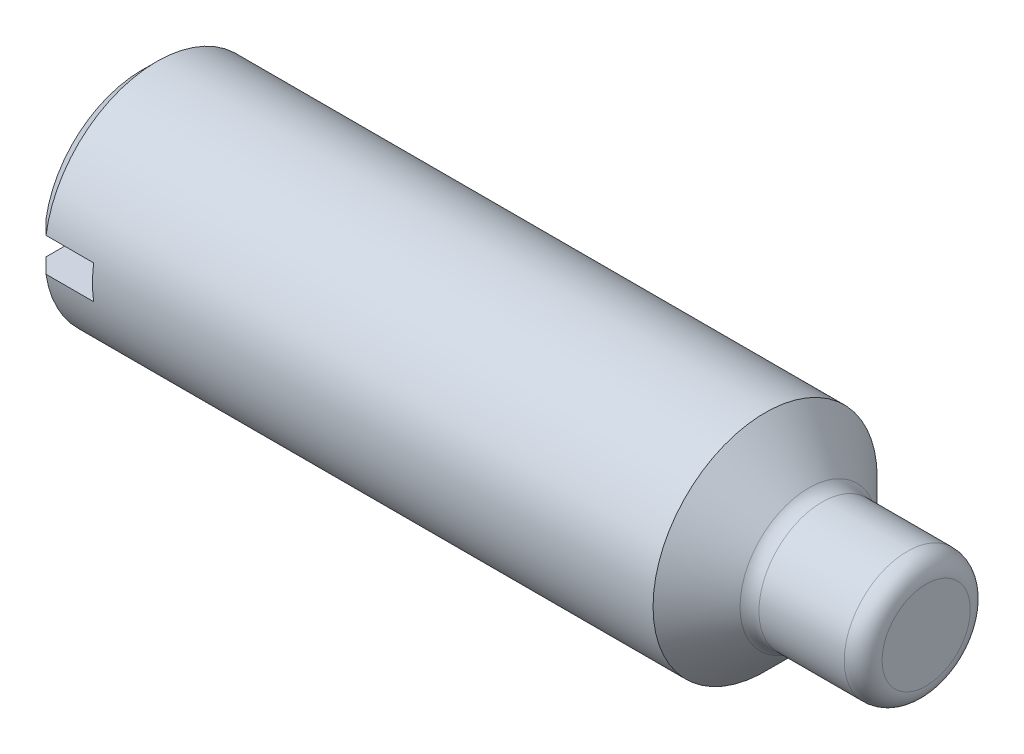
from build123d import *

# Parameters (mm, degrees)
SKETCH4_W          = 1.12
SKETCH4_H          = 0.6
CUT_EXTRUDE1_DEPTH = 50
FILLET1_R          = 0.3375


with BuildPart() as part:
    # Sketch3 → Base-Revolve (revolve)
    with BuildSketch(Plane.XY, mode=Mode.PRIVATE) as base_revolve_sk:
        Polygon((0, 0), (0, 1.732), (0.268, 2), (11.125, 2), (12, 1.125), (14, 1.125), (14, 0), align=None)
    revolve(base_revolve_sk.sketch.rotate(Axis((0, 0, 0), (1, 0, 0)), 90), axis=Axis((0, 0, 0), (1, 0, 0)))

    # Sketch4 → Cut-Extrude1 (cut, symmetric)
    with BuildSketch(Plane.XY):
        with Locations((0.56, 0)):
            Rectangle(SKETCH4_W, SKETCH4_H)
    extrude(amount=CUT_EXTRUDE1_DEPTH, both=True, mode=Mode.SUBTRACT)

    # Fillet1
    fillet1_edges = [part.edges().sort_by_distance(p)[0] for p in [
        (14, 0, -1.125),
        (12, 0, -1.125),
    ]]
    fillet(fillet1_edges, radius=FILLET1_R)


solid = part.part
